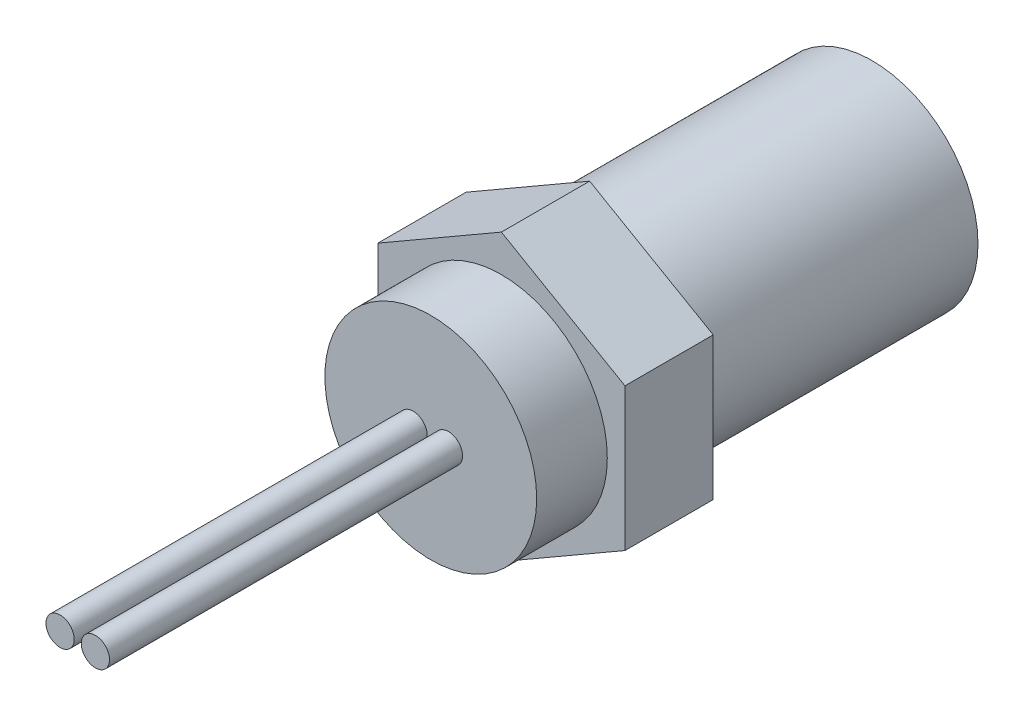
SolidWorks part; units mm, degrees
ref_plane "Front Plane" through (0, 0, 0) normal (0, 0, 1) x (1, 0, 0)
ref_plane "Top Plane" through (0, 0, 0) normal (0, 1, 0) x (1, 0, 0)
ref_plane "Right Plane" through (0, 0, 0) normal (1, 0, 0) x (0, 0, -1)
sketch "Sketch1" plane through (0, 0, 0) normal (0, 0, 1) x (1, 0, 0)
  circle A0 centre (0, 0) radius 3
  dimension "D1" = 6
extrude "Boss-Extrude1" add sketch "Sketch1" along normal blind 8
cosmetic thread "Cosmetic Thread1" parameters "D1"=8, "D2"=4.917
sketch "Sketch2" plane through (0, 0, 8) normal (0, 0, 1) x (1, 0, 0)
  line L1 (0, 4.0415) -> (-3.5, 2.0207)
  line L2 (-3.5, 2.0207) -> (-3.5, -2.0207)
  line L3 (-3.5, -2.0207) -> (0, -4.0415)
  line L4 (0, -4.0415) -> (3.5, -2.0207)
  line L5 (3.5, -2.0207) -> (3.5, 2.0207)
  line L6 (3.5, 2.0207) -> (0, 4.0415)
  circle A0 centre (0, 0) radius 3.5 construction
  dimension "D1" = 7
extrude "Boss-Extrude2" add sketch "Sketch2" along normal blind 2.5
sketch "Sketch3" plane through (0, 0, 10.5) normal (0, 0, 1) x (1, 0, 0)
  circle A0 centre (0, 0) radius 3
  dimension "D1" = 6
extrude "Boss-Extrude3" add sketch "Sketch3" along normal blind 2
sketch "Sketch4" plane through (0, 0, 12.5) normal (0, 0, 1) x (1, 0, 0)
  circle A0 centre (0.5, 0) radius 0.4
  circle A1 centre (-0.5, 0) radius 0.4
  dimension "D1" = 0.8
  dimension "D2" = 1
  dimension "D3" = 0.5
extrude "Boss-Extrude4" add sketch "Sketch4" along normal blind 10
